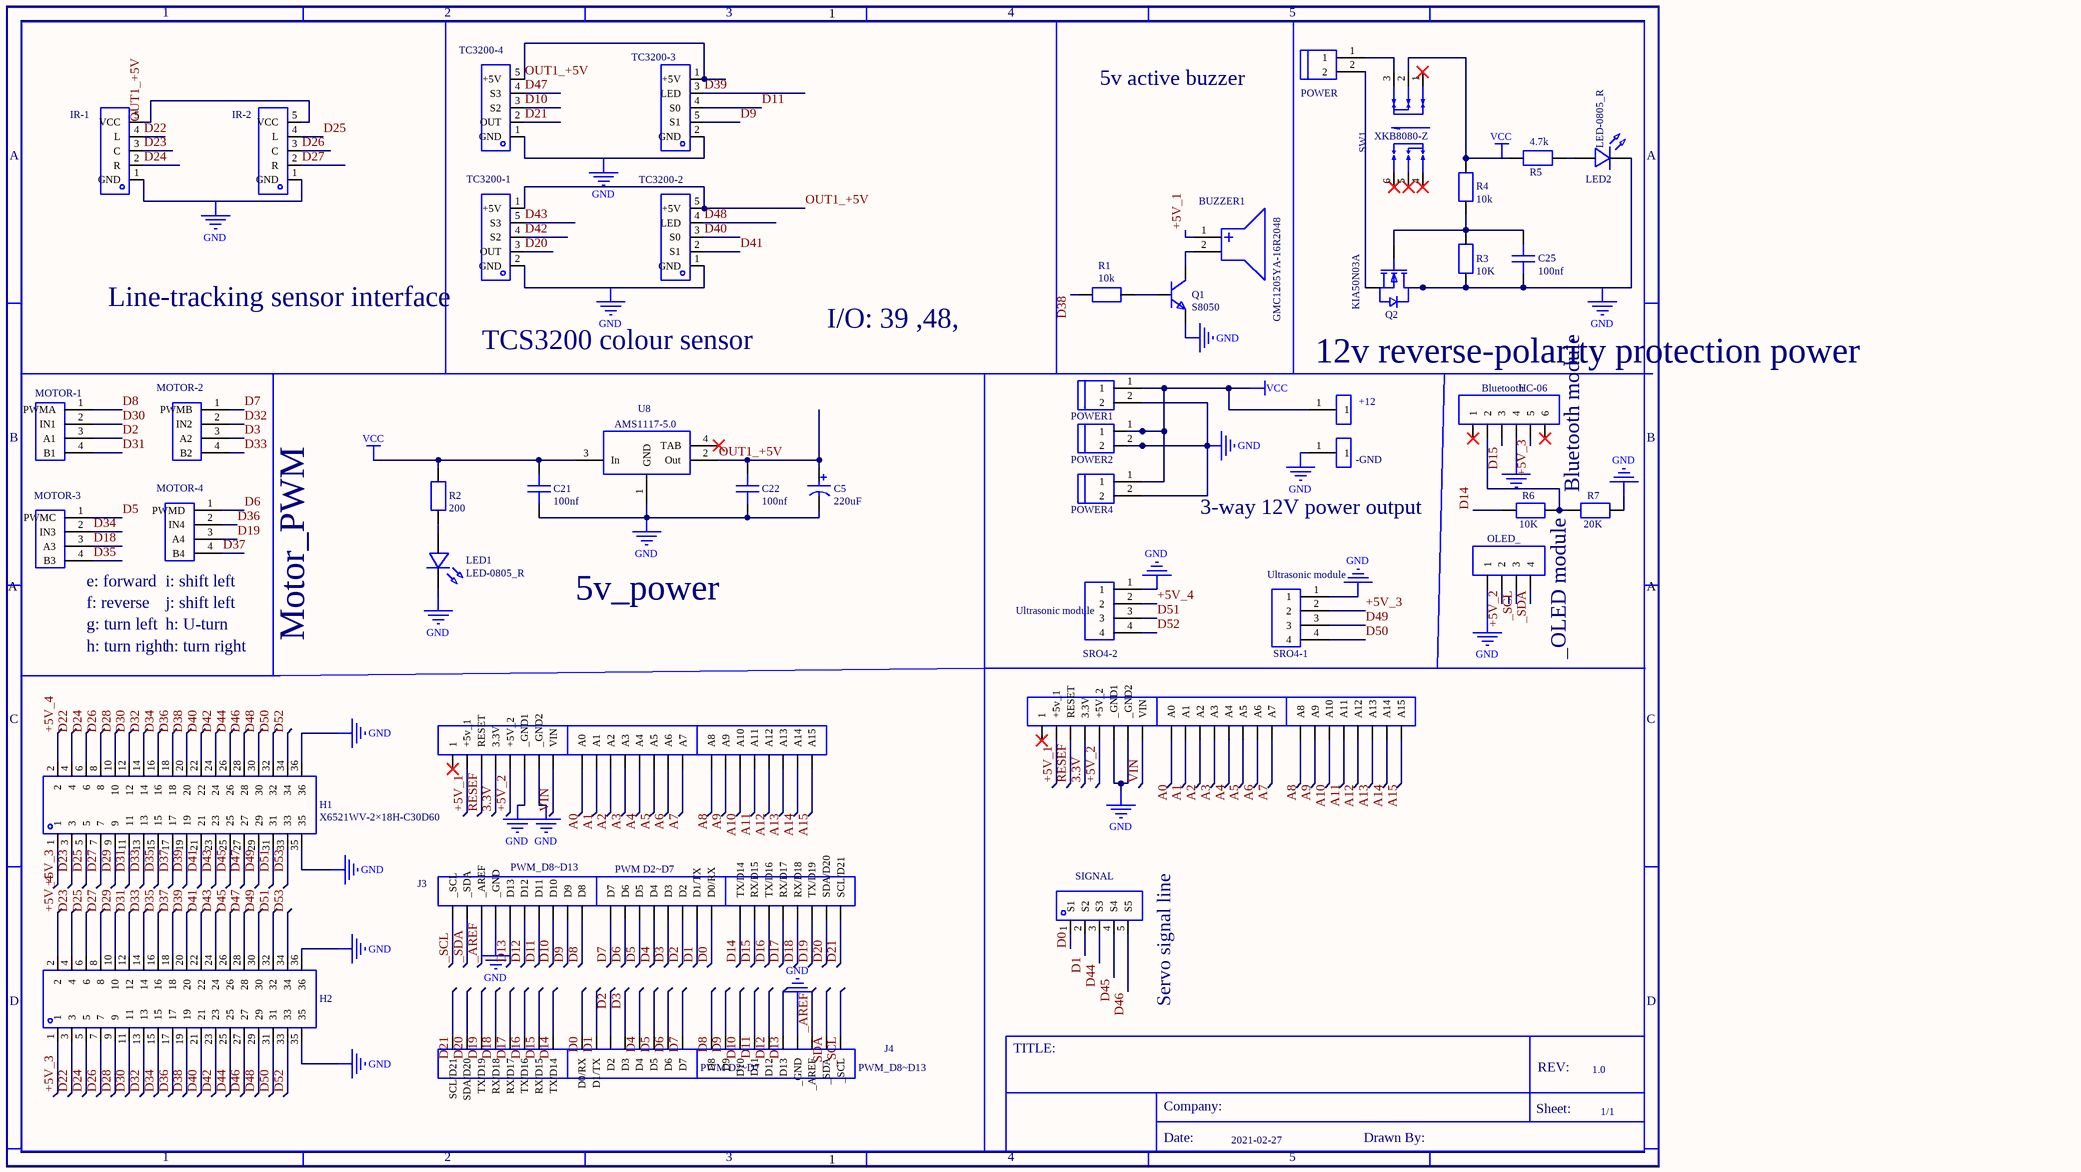
[diagram p0: MISC49934-3.schdoc]
# Altium project MISC49934-2.PrjPcb
1 sheet, 53 parts. Net scope: global (net labels, ports and power ports of the same name join across sheets).
Board file: MISC49934.pcbdoc

## Sheet MISC49934-3.schdoc
size 292 x 204 mm; Name: MISC49934; @Project Name: MISC49934; REV: 1.0; Date: 2021-02-27; Sheet: 1/1

### Parts
+12  Pad  [焊盘]  (value not drawn)
-GND  Pad  [焊盘]  (value not drawn)
BUZZER1  GMC1205YA-16R2048  [BUZ-TH_BD12.0-P6.50-D0.6-FD]
C5  220uF
C21  100nf  [C0603]
C22  100nf  [C0603]
C25  100nf  [C0603]
H1  X6521WV-2×18H-C30D60  [HDR-TH_36P-2.54-V-M-R2-C18-S2.54]
H2  X6521WV-2×18H-C30D60  [HDR-TH_36P-2.54-V-M-R2-C18-S2.54]  (value not drawn)
HC-06  Bluetooth  [HDR-F-2.54_1X6]
IR-1  XH-5A_C722874  [CONN-TH_XH-5A]  (value not drawn)
IR-2  XH-5A_C722874  [CONN-TH_XH-5A]  (value not drawn)
J1  3-way TX/RX  [HDR-M-2.54_1X8]  (value not drawn)
J2  PWM D2~D7  [HDR-M-2.54_1X8]
J3  PWM_D8~D13  [HDR-M-2.54_1X10]
J4  PWM_D8~D13  [HDR-M-2.54_1X10]
J5  PWM D2~D7  [HDR-M-2.54_1X8]
J6  3-way TX/RX  [HDR-M-2.54_1X8]  (value not drawn)
J7  HDR-M-2.54_1x8  [HDR-M-2.54_1X8]  (value not drawn)
J8  HDR-M-2.54_1x8  [HDR-M-2.54_1X8]  (value not drawn)
J9  HDR-M-2.54_1x8  [HDR-M-2.54_1X8]  (value not drawn)
J12  HDR-M-2.54_1x8  [HDR-M-2.54_1X8]  (value not drawn)
J13  HDR-M-2.54_1x8  [HDR-M-2.54_1X8]  (value not drawn)
J14  HDR-M-2.54_1x8  [HDR-M-2.54_1X8]  (value not drawn)
LED1  LED-0805_R  [LED0805_RED]
LED2  LED-0805_R  [LED0805_RED]
MOTOR-1  MOTOR-1  [CONN-TH_4P-P2.50_XH-4A]
MOTOR-2  MOTOR-2  [CONN-TH_4P-P2.50_XH-4A]  (value not drawn)
MOTOR-3  MOTOR-3  [CONN-TH_4P-P2.50_XH-4A]  (value not drawn)
MOTOR-4  MOTOR-4  [CONN-TH_4P-P2.50_XH-4A]  (value not drawn)
OLED-  OLED_  [HDR-F-2.54_1X4]
POWER  XH-2AW  [CONN-TH_2P-P2.50_XH-2AW]  (value not drawn)
POWER1  XH-2AW  [CONN-TH_2P-P2.50_XH-2AW]  (value not drawn)
POWER2  XH-2AW  [CONN-TH_2P-P2.50_XH-2AW]  (value not drawn)
POWER4  XH-2AW  [CONN-TH_2P-P2.50_XH-2AW]  (value not drawn)
Q1  S8050  [SOT-23-3_L2.9-W1.3-P1.90-LS2.4-BR]
Q2  KIA50N03A  [TO-252-2_L6.6-W6.1-P4.57-LS9.9-TL-CW]
R1  10k  [R0603]
R2  200  [R0603]
R3  10K  [R0603]
R4  10k  [R0603]
R5  4.7k  [R0603]
R6  10K  [R0603]
R7  20K  [R0603]
SIGNAL  XH-5A_C722874  [CONN-TH_XH-5A]  (value not drawn)
SRO4-1  Ultrasonic module  [CONN-TH_4P-P2.50_XH-4A]
SRO4-2  Ultrasonic module  [CONN-TH_4P-P2.50_XH-4A]
SW1  XKB8080-Z  [SW-TH_6P-L8.0-W8.0-P2.50]
TC3200-1  XH-5A_C722874  [CONN-TH_XH-5A]  (value not drawn)
TC3200-2  XH-5A_C722874  [CONN-TH_XH-5A]  (value not drawn)
TC3200-3  XH-5A_C722874  [CONN-TH_XH-5A]  (value not drawn)
TC3200-4  XH-5A_C722874  [CONN-TH_XH-5A]  (value not drawn)
U8  AMS1117-5.0  [SOT-223_L6.5-W3.5-P2.30-LS7.0-BR]

### Nets
GND: -GND.1 C5.2 C21.1 C22.1 C25.1 H1.35 H1.36 H2.35 H2.36 HC-06.4 IR-1.1(GND) IR-2.1(GND) J3.4(_GND) J4.4(_GND) J9.6(_GND1) J9.7(_GND2) J12.6(_GND1) J12.7(_GND2) LED1.2 LED2.2 OLED-.1 POWER1.2 POWER2.2 POWER4.2 Q1.2(E) Q2.2(D) R3.1 R7.1 SRO4-1.1 SRO4-2.1 TC3200-1.2(GND) TC3200-2.1(GND) TC3200-3.2(GND) TC3200-4.1(GND) U8.1(GND)
VCC: +12.1 C21.2 POWER1.1 POWER2.1 POWER4.1 R2.2 R4.1 R5.1 SW1.2 U8.3(In)
3.3V: J9.4(3.3V) J12.4(3.3V)
+5V_1: BUZZER1.1(+) J9.2(+5v_1) J12.2(+5v_1)
+5V_2: J9.5(+5V_2) J12.5(+5V_2) OLED-.2
+5V_3: H1.1 H2.1 HC-06.5 SRO4-1.2
+5V_4: H1.2 H2.2 SRO4-2.2
_AREF: J3.3(_AREF) J4.3(_AREF)
_SCL: J3.1(_SCL) J4.1(_SCL) OLED-.3
_SDA: J3.2(_SDA) J4.2(_SDA) OLED-.4
A0: J8.1(A0) J13.1(A0)
A1: J8.2(A1) J13.2(A1)
A2: J8.3(A2) J13.3(A2)
A3: J8.4(A3) J13.4(A3)
A4: J8.5(A4) J13.5(A4)
A5: J8.6(A5) J13.6(A5)
A6: J8.7(A6) J13.7(A6)
A7: J8.8(A7) J13.8(A7)
A8: J7.1(A8) J14.1(A8)
A9: J7.2(A9) J14.2(A9)
A10: J7.3(A10) J14.3(A10)
A11: J7.4(A11) J14.4(A11)
A12: J7.5(A12) J14.5(A12)
A13: J7.6(A13) J14.6(A13)
A14: J7.7(A14) J14.7(A14)
A15: J7.8(A15) J14.8(A15)
D0: J2.8(D0/RX) J5.8(D0/RX) SIGNAL.1(S1)
D1: J2.7(D1/TX) J5.7(D1/TX) SIGNAL.2(S2)
D2: J2.6(D2) J5.6(D2) MOTOR-1.3(A1)
D3: J2.5(D3) J5.5(D3) MOTOR-2.3(A2)
D4: J2.4(D4) J5.4(D4)
D5: J2.3(D5) J5.3(D5) MOTOR-3.1(PWMC)
D6: J2.2(D6) J5.2(D6) MOTOR-4.1(PWMD)
D7: J2.1(D7) J5.1(D7) MOTOR-2.1(PWMB)
D8: J3.10(D8) J4.10(D8) MOTOR-1.1(PWMA)
D9: J3.9(D9) J4.9(D9) TC3200-3.5(S1)
D10: J3.8(D10) J4.8(D10) TC3200-4.3(S2)
D11: J3.7(D11) J4.7(D11) TC3200-3.4(S0)
D12: J3.6(D12) J4.6(D12)
D13: J3.5(D13) J4.5(D13)
D14: J1.1(TX/D14) J6.1(TX/D14) R6.2
D15: HC-06.3 J1.2(RX/D15) J6.2(RX/D15)
D16: J1.3(TX/D16) J6.3(TX/D16)
D17: J1.4(RX/D17) J6.4(RX/D17)
D18: J1.5(RX/D18) J6.5(RX/D18) MOTOR-3.3(A3)
D19: J1.6(TX/D19) J6.6(TX/D19) MOTOR-4.3(A4)
D20: J1.7(SDA/D20) J6.7(SDA/D20) TC3200-1.3(OUT)
D21: J1.8(SCL/D21) J6.8(SCL/D21) TC3200-4.2(OUT)
D22: H1.4 H2.3 IR-1.4(L)
D23: H1.3 H2.4 IR-1.3(C)
D24: H1.6 H2.5 IR-1.2(R)
D25: H1.5 H2.6 IR-2.4(L)
D26: H1.8 H2.7 IR-2.3(C)
D27: H1.7 H2.8 IR-2.2(R)
D28: H1.10 H2.9
D29: H1.9 H2.10
D30: H1.12 H2.11 MOTOR-1.2(IN1)
D31: H1.11 H2.12 MOTOR-1.4(B1)
D32: H1.14 H2.13 MOTOR-2.2(IN2)
D33: H1.13 H2.14 MOTOR-2.4(B2)
D34: H1.16 H2.15 MOTOR-3.2(IN3)
D35: H1.15 H2.16 MOTOR-3.4(B3)
D36: H1.18 H2.17 MOTOR-4.2(IN4)
D37: H1.17 H2.18 MOTOR-4.4(B4)
D38: H1.20 H2.19 R1.1
D39: H1.19 H2.20 TC3200-3.3(LED)
D40: H1.22 H2.21 TC3200-2.3(S0)
D41: H1.21 H2.22 TC3200-2.2(S1)
D42: H1.24 H2.23 TC3200-1.4(S2)
D43: H1.23 H2.24 TC3200-1.5(S3)
D44: H1.26 H2.25 SIGNAL.3(S3)
D45: H1.25 H2.26 SIGNAL.4(S4)
D46: H1.28 H2.27 SIGNAL.5(S5)
D47: H1.27 H2.28 TC3200-4.4(S3)
D48: H1.30 H2.29 TC3200-2.4(LED)
D49: H1.29 H2.30 SRO4-1.3
D50: H1.32 H2.31 SRO4-1.4
D51: H1.31 H2.32 SRO4-2.3
D52: H1.34 H2.33 SRO4-2.4
D53: H1.33 H2.34
OUT1_+5V: C5.1 C22.2 IR-1.5(VCC) IR-2.5(VCC) TC3200-1.1(+5V) TC3200-2.5(+5V) TC3200-3.1(+5V) TC3200-4.5(+5V) U8.2(Out)
RESEF: J9.3(RESET) J12.3(RESET)
VIN: J9.8(VIN) J12.8(VIN)
NetBUZZER1_2: BUZZER1.2(-) Q1.3(C)
NetC25_2: C25.2 Q2.1(G) R3.2 R4.2
NetHC-06_2: HC-06.2 R6.1 R7.2
NetLED1_1: LED1.1 R2.1
NetLED2_1: LED2.1 R5.2
NetPOWER_1: POWER.1 SW1.3
NetPOWER_2: POWER.2 Q2.3(S)
NetQ1_1: Q1.1(B) R1.2

Not connected (* = marked no-connect by the designer): HC-06 1* 6*; J9 1*; J12 1*; SW1 1* 4* 5* 6*; U8 4(TAB)*

### Notes on the sheet
- 5v active buzzer
- (near TC3200-1) Line-tracking sensor interface
- I/O: 39 ,48,
- TCS3200 colour sensor
- 12v reverse-polarity protection power
- (near -GND) 3-way 12V power output
- Bluetooth module
- f: reverse
- e: forward
- (near MOTOR-4) i: shift left
- (near MOTOR-4) j: shift left
- 5v_power
- h: turn right
- g: turn left
- h: U-turn
- Motor_PWM
- _OLED module
- (near SIGNAL) Servo signal line
- 1
- 2
- 3
- 4
- 5
- A
- B
- C
- D
- TITLE:
- Company:
- Sheet:
- REV:
- 1.0
- 1/1
- Date:
- 2021-02-27
- Drawn By:

### Library data of the parts
+12 = 焊盘: Convert to PCB: yes; UniqueId: ggea270ad2503fae617; Origin Footprint: Pad; Device: Pad; Symbol: Pad; Add into BOM: yes; FootprintName: Pad
-GND = 焊盘: Convert to PCB: yes; UniqueId: gge5ae3374a470267ca; Origin Footprint: Pad; Device: Pad; Symbol: Pad; Add into BOM: yes; FootprintName: Pad
BUZZER1 = GMC1205YA-16R2048: Manufacturer: INGHAi; Convert to PCB: yes; UniqueId: gge6864b8a05df91b1c; Paste Type: expand; Origin Footprint: BUZ-TH_BD12.0-P6.50-D0.6-FD; Device: GMC1205YA-16R2048; Symbol: GMC1205YA-16R2048; Add into BOM: yes; Supplier: LCSC; SupplierPart: C252915; ManufacturerPart: GMC1205YA-16R2048; Assembly Type: manualWeld; FootprintName: BUZ-TH_BD12.0-P6.50-D0.6-FD
C5 = CK1A221M-CRE54: Manufacturer: SEMTECH; Origin Footprint: CAP-SMD_BD6.3-L6.6-W6.6-LS7.6-FD; Convert to PCB: yes; UniqueId: gge86c78eb3b1d63687; Device: CK1A221M-CRE54; Symbol: 220uF; Add into BOM: yes; Supplier: LCSC; ManufacturerPart: CK1A221M-CRE54; SupplierPart: C131157; JLCPCB Part Class: Extended Part
C21 = 100nf: Convert to PCB: yes; UniqueId: gge26881bc8621d2de8; Origin Footprint: C0603; Device: 100nf; Symbol: 100nf; Add into BOM: yes; FootprintName: C0603
C22 = 100nf: Convert to PCB: yes; UniqueId: ggeb634487bf266b2c7; Origin Footprint: C0603; Device: 100nf; Symbol: 100nf; Add into BOM: yes; FootprintName: C0603
C25 = 100nf: Convert to PCB: yes; UniqueId: gge832546f236980201; Origin Footprint: C0603; Device: 100nf; Symbol: 100nf; Add into BOM: yes; FootprintName: C0603
H1 = X6521WV-2×18H-C30D60: Manufacturer: XKB Connectivity; Convert to PCB: yes; UniqueId: gge659cdb978af65a32; Origin Footprint: HDR-TH_36P-2.54-V-M-R2-C18-S2.54; Device: X6521WV-2×18H-C30D60; Symbol: X6521WV-2×18H-C30D60; Add into BOM: yes; Supplier: LCSC; SupplierPart: C725890; ManufacturerPart: X6521WV-2×18H-C30D60; JLCPCB Part Class: Extended Part; FootprintName: HDR-TH_36P-2.54-V-M-R2-C18-S2.54
H2 = X6521WV-2×18H-C30D60: Manufacturer: XKB Connectivity; Convert to PCB: yes; UniqueId: gged0ecacb582d29ab1; Origin Footprint: HDR-TH_36P-2.54-V-M-R2-C18-S2.54; Device: X6521WV-2×18H-C30D60; Symbol: X6521WV-2×18H-C30D60; Add into BOM: yes; Supplier: LCSC; SupplierPart: C725890; ManufacturerPart: X6521WV-2×18H-C30D60; JLCPCB Part Class: Extended Part; FootprintName: HDR-TH_36P-2.54-V-M-R2-C18-S2.54
HC-06 = 蓝牙: Convert to PCB: yes; UniqueId: ggedee795e1ea8021ca; Origin Footprint: HDR-F-2.54_1X6; Device: Bluetooth; Symbol: Bluetooth; Add into BOM: yes; SupplierPart: C40877; Supplier: LCSC; FootprintName: HDR-F-2.54_1X6
IR-1 = XH-5A: Manufacturer: CAX; Convert to PCB: yes; UniqueId: ggef1d6fd578c18cf8c; Origin Footprint: CONN-TH_XH-5A; Device: XH-5A; Symbol: XH-5A_C722874; Add into BOM: yes; Supplier: LCSC; SupplierPart: C722874; ManufacturerPart: XH-5A; JLCPCB Part Class: Extended Part; FootprintName: CONN-TH_XH-5A
IR-2 = XH-5A: Manufacturer: CAX; Convert to PCB: yes; UniqueId: ggef9f736673b98cea9; Origin Footprint: CONN-TH_XH-5A; Device: XH-5A; Symbol: XH-5A_C722874; Add into BOM: yes; Supplier: LCSC; SupplierPart: C722874; ManufacturerPart: XH-5A; JLCPCB Part Class: Extended Part; FootprintName: CONN-TH_XH-5A
J1 = 3路TX/RX: Convert to PCB: yes; UniqueId: gge9dc4b7b1e30ce3fa; Origin Footprint: HDR-M-2.54_1X8; Device: 3-way TX/RX; Symbol: 3-way TX/RX; Add into BOM: yes; SupplierPart: C190820; Supplier: LCSC; FootprintName: HDR-M-2.54_1X8
J2 = PWM D2~D7: Convert to PCB: yes; UniqueId: gge9f655628bd203dcb; Origin Footprint: HDR-M-2.54_1X8; Device: PWM D2~D7; Symbol: PWM D2~D7; Add into BOM: yes; SupplierPart: C190820; Supplier: LCSC; FootprintName: HDR-M-2.54_1X8
J3 = PWM_D8~D13: Convert to PCB: yes; UniqueId: gge25734fb99099d70d; Origin Footprint: HDR-M-2.54_1X10; Device: PWM_D8~D13; Symbol: PWM_D8~D13; Add into BOM: yes; SupplierPart: C57369; Supplier: LCSC; FootprintName: HDR-M-2.54_1X10
J4 = PWM_D8~D13: Convert to PCB: yes; UniqueId: gge9ab53663eb6b2481; Origin Footprint: HDR-M-2.54_1X10; Device: PWM_D8~D13; Symbol: PWM_D8~D13; Add into BOM: yes; SupplierPart: C57369; Supplier: LCSC; FootprintName: HDR-M-2.54_1X10
J5 = PWM D2~D7: Convert to PCB: yes; UniqueId: gge2d54ea47b229c178; Origin Footprint: HDR-M-2.54_1X8; Device: PWM D2~D7; Symbol: PWM D2~D7; Add into BOM: yes; SupplierPart: C190820; Supplier: LCSC; FootprintName: HDR-M-2.54_1X8
J6 = 3路TX/RX: Convert to PCB: yes; UniqueId: gge83e96a870e789e2a; Origin Footprint: HDR-M-2.54_1X8; Device: 3-way TX/RX; Symbol: 3-way TX/RX; Add into BOM: yes; SupplierPart: C190820; Supplier: LCSC; FootprintName: HDR-M-2.54_1X8
J7 = HDR-M-2.54_1x8: Convert to PCB: yes; UniqueId: ggef8426f22945a00d2; Origin Footprint: HDR-M-2.54_1X8; Device: HDR-M-2.54_1x8; Symbol: HDR-M-2.54_1x8; Add into BOM: yes; SupplierPart: C190820; Supplier: LCSC; FootprintName: HDR-M-2.54_1X8
J8 = HDR-M-2.54_1x8: Convert to PCB: yes; UniqueId: gge9b77a95cd2a4dd53; Origin Footprint: HDR-M-2.54_1X8; Device: HDR-M-2.54_1x8; Symbol: HDR-M-2.54_1x8; Add into BOM: yes; SupplierPart: C190820; Supplier: LCSC; FootprintName: HDR-M-2.54_1X8
J9 = HDR-M-2.54_1x8: Convert to PCB: yes; UniqueId: ggea99c644f7a9f27b0; Origin Footprint: HDR-M-2.54_1X8; Device: HDR-M-2.54_1x8; Symbol: HDR-M-2.54_1x8; Add into BOM: yes; SupplierPart: C190820; Supplier: LCSC; FootprintName: HDR-M-2.54_1X8
J12 = HDR-M-2.54_1x8: Convert to PCB: yes; UniqueId: ggea33f8713a29a63ab; Origin Footprint: HDR-M-2.54_1X8; Device: HDR-M-2.54_1x8; Symbol: HDR-M-2.54_1x8; Add into BOM: yes; SupplierPart: C190820; Supplier: LCSC; FootprintName: HDR-M-2.54_1X8
J13 = HDR-M-2.54_1x8: Convert to PCB: yes; UniqueId: ggec004e3960c01b6de; Origin Footprint: HDR-M-2.54_1X8; Device: HDR-M-2.54_1x8; Symbol: HDR-M-2.54_1x8; Add into BOM: yes; SupplierPart: C190820; Supplier: LCSC; FootprintName: HDR-M-2.54_1X8
J14 = HDR-M-2.54_1x8: Convert to PCB: yes; UniqueId: gge9469fb26cc561a9c; Origin Footprint: HDR-M-2.54_1X8; Device: HDR-M-2.54_1x8; Symbol: HDR-M-2.54_1x8; Add into BOM: yes; SupplierPart: C190820; Supplier: LCSC; FootprintName: HDR-M-2.54_1X8
LED1 = 17-21SURC/S530-A3/TR8: Manufacturer: EVERLIGHT(台湾亿光); Convert to PCB: yes; UniqueId: ggec732b67aada0fc10; Origin Footprint: LED0805_RED; Device: 17-21SURC/S530-A3/TR8; Symbol: LED-0805_R; Add into BOM: yes; ManufacturerPart: 17-21SURC/S530-A3/TR8; SupplierPart: C72037; FootprintName: LED0805_RED
LED2 = 17-21SURC/S530-A3/TR8: Manufacturer: EVERLIGHT(台湾亿光); Convert to PCB: yes; UniqueId: ggef125ffb01255ffaa; Origin Footprint: LED0805_RED; Device: 17-21SURC/S530-A3/TR8; Symbol: LED-0805_R; Add into BOM: yes; ManufacturerPart: 17-21SURC/S530-A3/TR8; SupplierPart: C72037; FootprintName: LED0805_RED
MOTOR-1 = XH-4A: Manufacturer: BOOMELE; Convert to PCB: yes; UniqueId: gge8ad8ee00da7474c6; Paste Type: expand; Origin Footprint: CONN-TH_4P-P2.50_XH-4A; Device: XH-4A; Symbol: MOTOR-1; image: C37815.jpg; Add into BOM: yes; Supplier: LCSC; ManufacturerPart: XH-4A; SupplierPart: C37815; FootprintName: CONN-TH_4P-P2.50_XH-4A
MOTOR-2 = XH-4A: Manufacturer: BOOMELE; Convert to PCB: yes; UniqueId: gge1a2eb5d5367d2aea; Paste Type: expand; Origin Footprint: CONN-TH_4P-P2.50_XH-4A; Device: XH-4A; Symbol: MOTOR-2; image: C37815.jpg; Add into BOM: yes; Supplier: LCSC; ManufacturerPart: XH-4A; SupplierPart: C37815; FootprintName: CONN-TH_4P-P2.50_XH-4A
MOTOR-3 = XH-4A: Manufacturer: BOOMELE; Convert to PCB: yes; UniqueId: gge8a46302927414b47; Paste Type: expand; Origin Footprint: CONN-TH_4P-P2.50_XH-4A; Device: XH-4A; Symbol: MOTOR-3; image: C37815.jpg; Add into BOM: yes; Supplier: LCSC; ManufacturerPart: XH-4A; SupplierPart: C37815; FootprintName: CONN-TH_4P-P2.50_XH-4A
MOTOR-4 = XH-4A: Manufacturer: BOOMELE; Convert to PCB: yes; UniqueId: ggee8d01e52059145f6; Paste Type: expand; Origin Footprint: CONN-TH_4P-P2.50_XH-4A; Device: XH-4A; Symbol: MOTOR-4; image: C37815.jpg; Add into BOM: yes; Supplier: LCSC; ManufacturerPart: XH-4A; SupplierPart: C37815; FootprintName: CONN-TH_4P-P2.50_XH-4A
OLED- = OLED_: Convert to PCB: yes; UniqueId: ggec9b55ab8fdae2c39; Origin Footprint: HDR-F-2.54_1X4; Device: OLED_; Symbol: OLED_; Add into BOM: yes; SupplierPart: C225501; Supplier: LCSC; FootprintName: HDR-F-2.54_1X4
POWER = XH-2AW: Manufacturer: BOOMELE; Convert to PCB: yes; UniqueId: gge8d4318519d7c15a8; Origin Footprint: CONN-TH_2P-P2.50_XH-2AW; Device: XH-2AW; Symbol: XH-2AW; Add into BOM: yes; Supplier: LCSC; ManufacturerPart: XH-2AW; SupplierPart: C33132; JLCPCB Part Class: Extended Part; FootprintName: CONN-TH_2P-P2.50_XH-2AW
POWER1 = XH-2AW: Manufacturer: BOOMELE; Convert to PCB: yes; UniqueId: gge1b7117180344bd75; Origin Footprint: CONN-TH_2P-P2.50_XH-2AW; Device: XH-2AW; Symbol: XH-2AW; Add into BOM: yes; Supplier: LCSC; ManufacturerPart: XH-2AW; SupplierPart: C33132; JLCPCB Part Class: Extended Part; FootprintName: CONN-TH_2P-P2.50_XH-2AW
POWER2 = XH-2AW: Manufacturer: BOOMELE; Convert to PCB: yes; UniqueId: ggebc0f2800e842d02f; Origin Footprint: CONN-TH_2P-P2.50_XH-2AW; Device: XH-2AW; Symbol: XH-2AW; Add into BOM: yes; Supplier: LCSC; ManufacturerPart: XH-2AW; SupplierPart: C33132; JLCPCB Part Class: Extended Part; FootprintName: CONN-TH_2P-P2.50_XH-2AW
POWER4 = XH-2AW: Manufacturer: BOOMELE; Convert to PCB: yes; UniqueId: ggea5c9b238aa5ea54b; Origin Footprint: CONN-TH_2P-P2.50_XH-2AW; Device: XH-2AW; Symbol: XH-2AW; Add into BOM: yes; Supplier: LCSC; ManufacturerPart: XH-2AW; SupplierPart: C33132; JLCPCB Part Class: Extended Part; FootprintName: CONN-TH_2P-P2.50_XH-2AW
Q1 = S8050: Manufacturer: WPMtek(维攀微); Convert to PCB: yes; UniqueId: gged639cbb8b6e81ceb; Origin Footprint: SOT-23-3_L2.9-W1.3-P1.90-LS2.4-BR; Device: S8050; Symbol: S8050; Add into BOM: yes; Supplier: LCSC; SupplierPart: C2688231; ManufacturerPart: S8050; FootprintName: SOT-23-3_L2.9-W1.3-P1.90-LS2.4-BR
Q2 = KIA50N03A: Manufacturer: KIA; Convert to PCB: yes; UniqueId: gge62ad891af4153567; Paste Type: recommend; Origin Footprint: TO-252-2_L6.6-W6.1-P4.57-LS9.9-TL-CW; Device: KIA50N03A; Symbol: KIA50N03A; Add into BOM: yes; Supplier: LCSC; ManufacturerPart: KIA50N03A; SupplierPart: C112249; FootprintName: TO-252-2_L6.6-W6.1-P4.57-LS9.9-TL-CW
R1 = 10k: Convert to PCB: yes; UniqueId: gge7880bea439704250; Origin Footprint: R0603; Device: 10k; Symbol: 10k; Add into BOM: yes; FootprintName: R0603
R2 = 200: Convert to PCB: yes; UniqueId: ggeb60cf776bd432245; Origin Footprint: R0603; Device: 200; Symbol: 200; Add into BOM: yes; FootprintName: R0603
R3 = 10K: Convert to PCB: yes; UniqueId: ggea893674240a93232; Origin Footprint: R0603; Device: 10K; Symbol: 10K; Add into BOM: yes; FootprintName: R0603
R4 = 10k: Convert to PCB: yes; UniqueId: gge95672fead64f669b; Origin Footprint: R0603; Device: 10k; Symbol: 10k; Add into BOM: yes; FootprintName: R0603
R5 = 4.7k: Convert to PCB: yes; UniqueId: ggeb921592e8123472b; Origin Footprint: R0603; Device: 4.7k; Symbol: 4.7k; Add into BOM: yes; FootprintName: R0603
R6 = 10K: Convert to PCB: yes; UniqueId: ggea09e557dc4b0f267; Origin Footprint: R0603; Device: 10K; Symbol: 10K; Add into BOM: yes; FootprintName: R0603
R7 = 20K: Convert to PCB: yes; UniqueId: ggefa87d43415f6fba4; Origin Footprint: R0603; Device: 20K; Symbol: 20K; Add into BOM: yes; FootprintName: R0603
SIGNAL = XH-5A: Manufacturer: CAX; Convert to PCB: yes; UniqueId: ggef25d8ad3b6dbff6c; Origin Footprint: CONN-TH_XH-5A; Device: XH-5A; Symbol: XH-5A_C722874; Add into BOM: yes; Supplier: LCSC; SupplierPart: C722874; ManufacturerPart: XH-5A; JLCPCB Part Class: Extended Part; FootprintName: CONN-TH_XH-5A
SRO4-1 = XH-4A: Manufacturer: BOOMELE; Convert to PCB: yes; UniqueId: gged0cae50b5c4ca524; Paste Type: expand; Origin Footprint: CONN-TH_4P-P2.50_XH-4A; Device: XH-4A; Symbol: Ultrasonic module; image: C37815.jpg; Add into BOM: yes; Supplier: LCSC; ManufacturerPart: XH-4A; SupplierPart: C37815; FootprintName: CONN-TH_4P-P2.50_XH-4A
SRO4-2 = XH-4A: Manufacturer: BOOMELE; Convert to PCB: yes; UniqueId: ggea43ed68f5d678f1e; Paste Type: expand; Origin Footprint: CONN-TH_4P-P2.50_XH-4A; Device: XH-4A; Symbol: Ultrasonic module; image: C37815.jpg; Add into BOM: yes; Supplier: LCSC; ManufacturerPart: XH-4A; SupplierPart: C37815; FootprintName: CONN-TH_4P-P2.50_XH-4A
SW1 = XKB8080-Z: Manufacturer: XKB Enterprise; Convert to PCB: yes; UniqueId: ggebeca442f7afc0640; Paste Type: expand; Origin Footprint: SW-TH_6P-L8.0-W8.0-P2.50; Device: XKB8080-Z; Symbol: XKB8080-Z; Add into BOM: yes; Supplier: LCSC; SupplierPart: C318860; ManufacturerPart: XKB8080-Z; FootprintName: SW-TH_6P-L8.0-W8.0-P2.50
TC3200-1 = XH-5A: Manufacturer: CAX; Convert to PCB: yes; UniqueId: gge71b1515a8a211d92; Origin Footprint: CONN-TH_XH-5A; Device: XH-5A; Symbol: XH-5A_C722874; Add into BOM: yes; Supplier: LCSC; SupplierPart: C722874; ManufacturerPart: XH-5A; JLCPCB Part Class: Extended Part; FootprintName: CONN-TH_XH-5A
TC3200-2 = XH-5A: Manufacturer: CAX; Convert to PCB: yes; UniqueId: gge72e8df8b984ab8d8; Origin Footprint: CONN-TH_XH-5A; Device: XH-5A; Symbol: XH-5A_C722874; Add into BOM: yes; Supplier: LCSC; SupplierPart: C722874; ManufacturerPart: XH-5A; JLCPCB Part Class: Extended Part; FootprintName: CONN-TH_XH-5A
TC3200-3 = XH-5A: Manufacturer: CAX; Convert to PCB: yes; UniqueId: gge9fdf798649146c21; Origin Footprint: CONN-TH_XH-5A; Device: XH-5A; Symbol: XH-5A_C722874; Add into BOM: yes; Supplier: LCSC; SupplierPart: C722874; ManufacturerPart: XH-5A; JLCPCB Part Class: Extended Part; FootprintName: CONN-TH_XH-5A
TC3200-4 = XH-5A: Manufacturer: CAX; Convert to PCB: yes; UniqueId: ggea7c7524e2f0bfc69; Origin Footprint: CONN-TH_XH-5A; Device: XH-5A; Symbol: XH-5A_C722874; Add into BOM: yes; Supplier: LCSC; SupplierPart: C722874; ManufacturerPart: XH-5A; JLCPCB Part Class: Extended Part; FootprintName: CONN-TH_XH-5A
U8 = AMS1117-5.0: Manufacturer: AMS; Convert to PCB: yes; UniqueId: ggeba0b5f381eb36d62; Paste Type: base; Origin Footprint: SOT-223_L6.5-W3.5-P2.30-LS7.0-BR; Device: AMS1117-5.0; Symbol: AMS1117-5.0; image: C6187.jpg; Add into BOM: yes; Supplier: LCSC; ManufacturerPart: AMS1117-5.0; SupplierPart: C6187; FootprintName: SOT-223_L6.5-W3.5-P2.30-LS7.0-BR